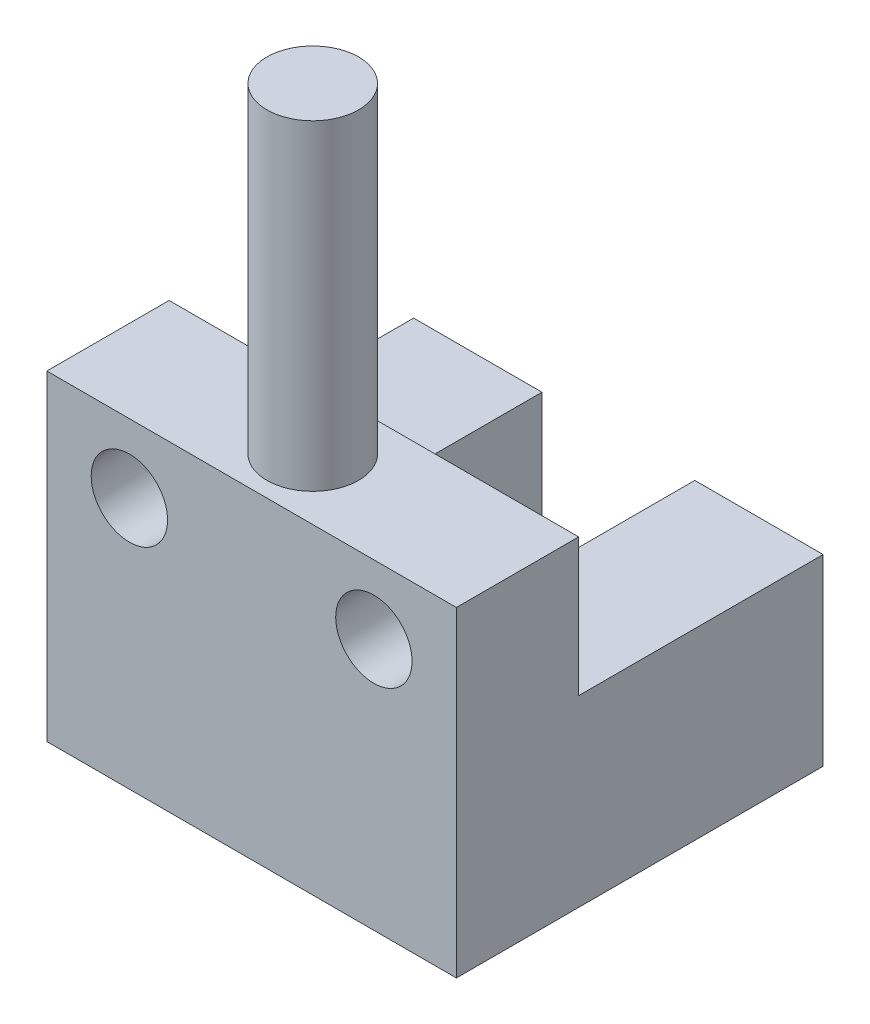
from build123d import *

# Parameters (mm, degrees)
BOSS_EXTRUDE1_DEPTH = 6
SKETCH2_W           = 13.4
SKETCH2_H           = 4
BOSS_EXTRUDE2_DEPTH = 4.5
SKETCH3_R           = 1.5
BOSS_EXTRUDE3_DEPTH = 10.5
SKETCH4_R           = 1.25
CUT_EXTRUDE1_DEPTH  = 10.5
SKETCH5_R           = 0.5
BOSS_EXTRUDE4_DEPTH = 5


with BuildPart() as part:
    # Sketch1 → Boss-Extrude1 (new body)
    with BuildSketch(Plane(origin=(0, 0, 0), x_dir=(1, 0, 0), z_dir=(0, 1, 0))):
        Polygon((2.5, 6), (6.7, 6), (6.7, -6), (-6.7, -6), (-6.7, 6), (-2.5, 6), (-2.5, 0.5), (2.5, 0.5), align=None)
    extrude(amount=BOSS_EXTRUDE1_DEPTH)

    # Sketch2 → Boss-Extrude2 (add)
    with BuildSketch(Plane(origin=(0, 6, 0), x_dir=(1, 0, 0), z_dir=(0, 1, 0))):
        with Locations((0, -4)):
            Rectangle(SKETCH2_W, SKETCH2_H)
    extrude(amount=BOSS_EXTRUDE2_DEPTH)

    # Sketch3 → Boss-Extrude3 (add)
    with BuildSketch(Plane(origin=(0, 10.5, 0), x_dir=(1, 0, 0), z_dir=(0, 1, 0))):
        with Locations(Location((0, -4, 0), (0, 0, 90))):
            Circle(SKETCH3_R)
    extrude(amount=BOSS_EXTRUDE3_DEPTH)

    # Sketch4 → Cut-Extrude1 (cut)
    with BuildSketch(Plane(origin=(0, 0, 2), x_dir=(-1, 0, 0), z_dir=(0, 0, -1))):
        with Locations((-4, 8.25)):
            Circle(SKETCH4_R)
        with Locations((4, 8.25)):
            Circle(SKETCH4_R)
    extrude(amount=-CUT_EXTRUDE1_DEPTH, mode=Mode.SUBTRACT)

    # Sketch5 → Boss-Extrude4 (add)
    with BuildSketch(Plane.ZY.offset(-2.5)):
        with Locations(Location((-4, 3, 0), (0, 0, 180))):
            Circle(SKETCH5_R)
    extrude(amount=BOSS_EXTRUDE4_DEPTH)


solid = part.part
